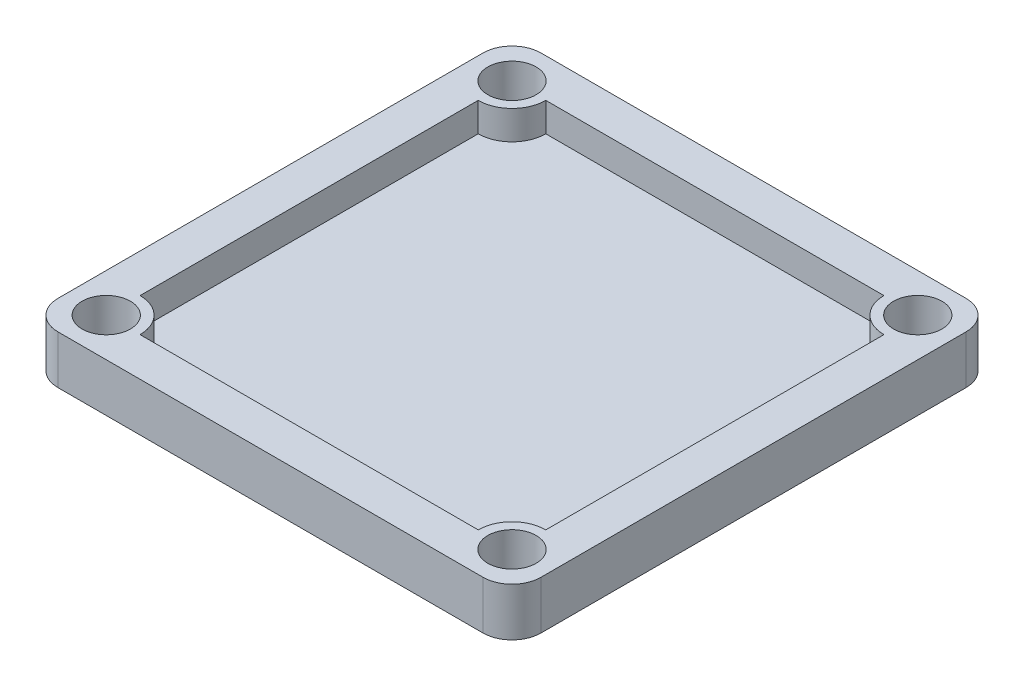
SolidWorks part; units mm, degrees
ref_plane "Front Plane" through (0, 0, 0) normal (0, 0, 1) x (1, 0, 0)
ref_plane "Top Plane" through (0, 0, 0) normal (0, 1, 0) x (1, 0, 0)
ref_plane "Right Plane" through (0, 0, 0) normal (1, 0, 0) x (0, 0, -1)
sketch "Sketch1" plane through (0, 0, 0) normal (0, 1, 0) x (1, 0, 0)
  line L1 (-220, -250) -> (220, -250)
  line L2 (-250, -220) -> (-250, 220)
  line L3 (-220, 250) -> (220, 250)
  line L4 (250, -220) -> (250, 220)
  line L5 (-250, -250) -> (250, 250) construction
  line L6 (-250, 250) -> (250, -250) construction
  arc A0 (-220, -250) -> (-250, -220) centre (-220, -220) cw
  arc A1 (-250, 220) -> (-220, 250) centre (-220, 220) cw
  arc A2 (250, 220) -> (220, 250) centre (220, 220) ccw
  arc A3 (220, -250) -> (250, -220) centre (220, -220) ccw
  point P0 (0, 0)
  dimension "D1" = 30
  dimension "D2" = 30
  dimension "D3" = 30
  dimension "D4" = 30
  dimension "D5" = 500
  dimension "D6" = 500
extrude "Boss-Extrude1" add sketch "Sketch1" along normal blind 50
sketch "Sketch2" plane through (0, 50, 0) normal (0, 1, 0) x (1, 0, 0)
  line L0 (-372.8708, 0) -> (441.5882, 0) construction
  line L5 (0, 411.5244) -> (0, -340.5073) construction
  line L7 (-175, -210) -> (175, -210)
  line L8 (-210, -175) -> (-210, 175)
  line L9 (-175, 210) -> (175, 210)
  line L10 (210, -175) -> (210, 175)
  line L11 (-210, -210) -> (210, 210) construction
  line L12 (-210, 210) -> (210, -210) construction
  arc A1 (175, 210) -> (210, 175) centre (210, 210) ccw
  arc A3 (-175, 210) -> (-210, 175) centre (-210, 210) cw
  arc A8 (175, -210) -> (210, -175) centre (210, -210) cw
  arc A9 (-175, -210) -> (-210, -175) centre (-210, -210) ccw
  point P4 (0, 0)
  dimension "D1" = 420
  dimension "D2" = 420
extrude "Cut-Extrude1" cut sketch "Sketch2" against normal blind 30
sketch "Sketch3" plane through (0, 50, 0) normal (0, 1, 0) x (1, 0, 0)
  line L0 (-471.3549, 0) -> (455.5106, 0) construction
  line L1 (0, 559.6412) -> (0, -544.8116) construction
  circle A0 centre (-210, 210) radius 25
  circle A2 centre (210, 210) radius 25
  circle A3 centre (210, -210) radius 25
  circle A4 centre (-210, -210) radius 25
  dimension "D1" = 210
  dimension "D2" = 210
extrude "Cut-Extrude2" cut sketch "Sketch3" against normal up to next
